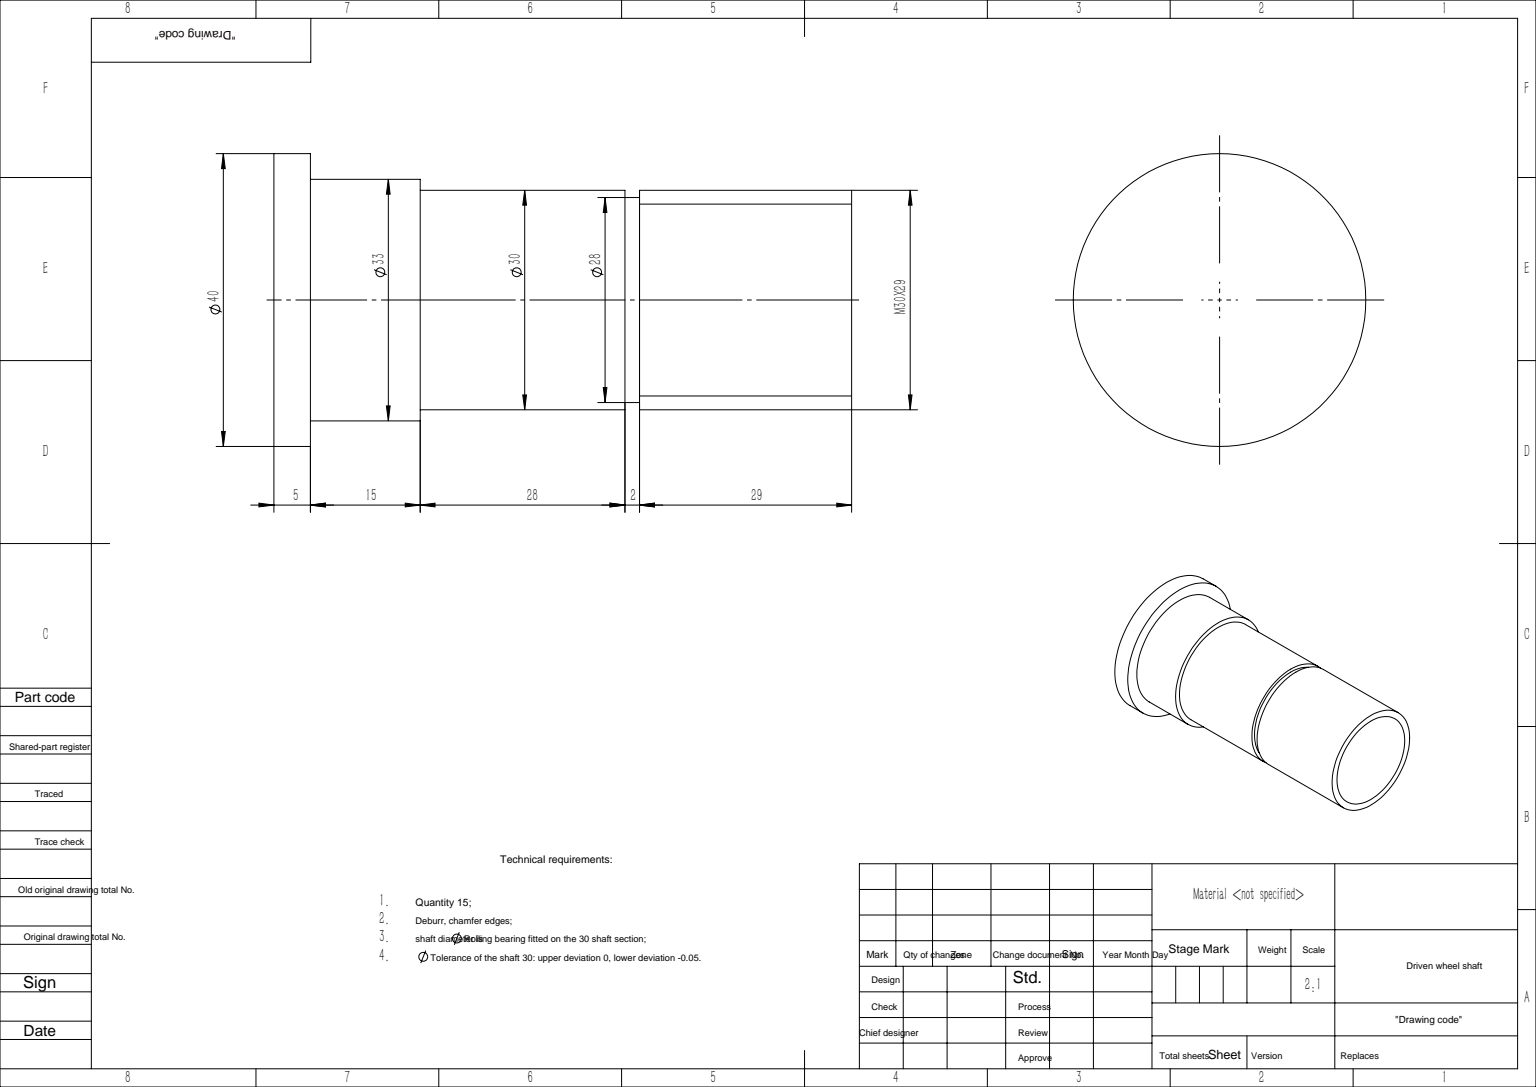
from build123d import *

# Parameters (mm, degrees)
CUT_EXTRUDE_START   = -29
SKETCH_3_R          = 15
SKETCH_3_R_2        = 14
CUT_EXTRUDE_1_DEPTH = 2


with BuildPart() as part:
    # 草图1 → 旋转1 (revolve)
    with BuildSketch(Plane.XY, mode=Mode.PRIVATE) as revolve_1_sk:
        Polygon((0, 0), (0, 20), (5, 20), (5, 16.5), (20, 16.5), (20, 15), (79, 15), (79, 0), align=None)
    revolve(revolve_1_sk.sketch.rotate(Axis((79, 0, 0), (-1, 0, 0)), 90), axis=Axis((79, 0, 0), (-1, 0, 0)))

    # 草图3 → 切除-拉伸1 (cut)
    with BuildSketch(Plane(origin=(79, 0, 0), x_dir=(0, 0, -1), z_dir=(1, 0, 0)).offset(CUT_EXTRUDE_START)):
        Circle(SKETCH_3_R)
        with Locations(Location((0, 0, 0), (0, 0, 90))):
            Circle(SKETCH_3_R_2, mode=Mode.SUBTRACT)
    extrude(amount=-CUT_EXTRUDE_1_DEPTH, mode=Mode.SUBTRACT)


solid = part.part
